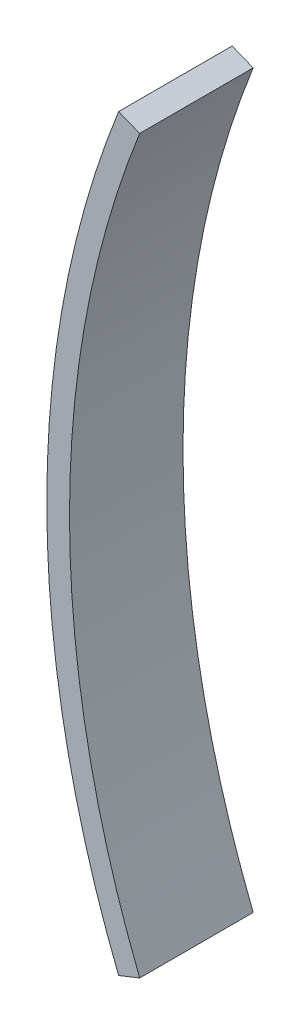
SolidWorks part; units mm, degrees
ref_plane "Front Plane" through (0, 0, 0) normal (0, 0, 1) x (1, 0, 0)
ref_plane "Top Plane" through (0, 0, 0) normal (0, 1, 0) x (1, 0, 0)
ref_plane "Right Plane" through (0, 0, 0) normal (1, 0, 0) x (0, 0, -1)
sketch "Sketch1" plane through (0, 0, 0) normal (0, 0, 1) x (1, 0, 0)
  line L0 (0, 0) -> (-503.6147, 0) construction
  line L1 (-298.5121, 102.31) -> (-187.8243, 102.31) construction
  line L2 (-298.5121, -102.31) -> (-187.8243, -102.31) construction
  line L3 (-256.7138, 102.31) -> (-262.6126, 104.6609)
  line L4 (-256.7138, -102.31) -> (-262.6126, -104.6609)
  arc A0 (-256.7138, 102.31) -> (-256.7138, -102.31) centre (0, 0) ccw
  arc A1 (-262.6126, 104.6609) -> (-262.6126, -104.6609) centre (0, 0) ccw
  dimension "D1" = 552.7
  dimension "D2" = 6.35
  dimension "D3" = 102.31
extrude "Boss-Extrude1" add sketch "Sketch1" along normal blind 31.75
